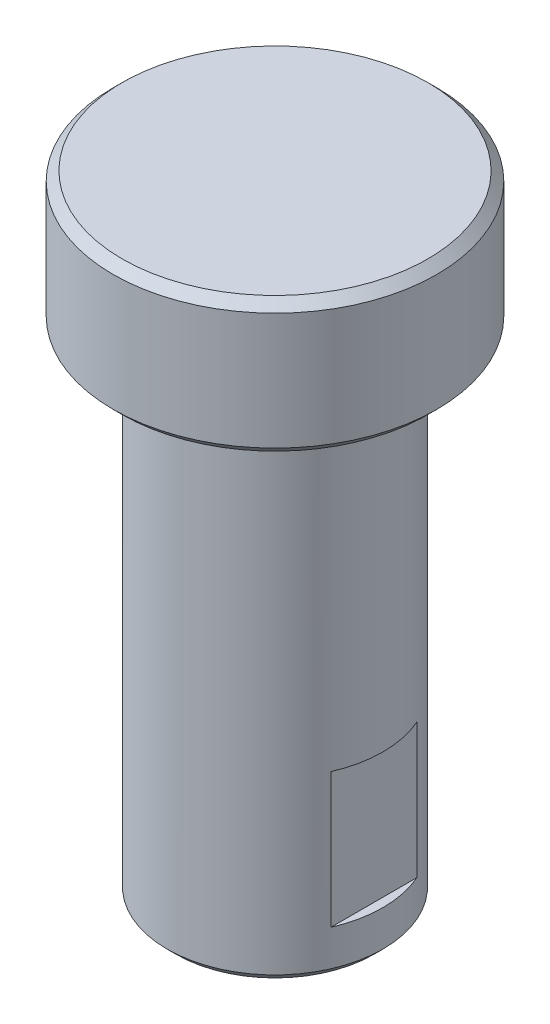
from build123d import *

# Parameters (mm, degrees)
CHAMFER1_SIZE              = 1
CUT_EXTRUDE1_DEPTH         = 55.911039474
CUT_EXTRUDE1_DEPTH_BACK    = 55.911039474
SKETCH3_W                  = 1
SKETCH3_H                  = 15
M14X1_5_TAPPED_HOLE1_D     = 12.5
M14X1_5_TAPPED_HOLE1_DEPTH = 20
M14X1_5_TAPPED_HOLE1_TIP   = 3.755378869


with BuildPart() as part:
    # Sketch2 → Revolve1 (revolve)
    with BuildSketch(Plane.XY, mode=Mode.PRIVATE) as revolve1_sk:
        Polygon((0, 48.654108317), (-18, 48.654108317), (-18, 33.654108317), (-12, 33.654108317), (-12, -21.345891683), (0, -21.345891683), align=None)
    revolve(revolve1_sk.sketch.rotate(Axis((0, 14.106387272, 0), (0, -1, 0)), 270), axis=Axis((0, 14.106387272, 0), (0, -1, 0)))

    # Chamfer1
    chamfer1_edges = [part.edges().sort_by_distance(p)[0] for p in [
        (0, -21.345891683, -12),
        (0, 33.654108317, -18),
        (0, 48.654108317, -18),
    ]]
    chamfer(chamfer1_edges, length=CHAMFER1_SIZE)

    # Sketch3 → Cut-Extrude1 (cut, two sides: drawn at the far end of the back side and taken through both)
    with BuildSketch(Plane.XY.offset(-CUT_EXTRUDE1_DEPTH_BACK)):
        with Locations((-11.5, -8.845891683)):
            Rectangle(SKETCH3_W, SKETCH3_H)
        with Locations((11.5, -8.845891683)):
            Rectangle(SKETCH3_W, SKETCH3_H)
    extrude(amount=CUT_EXTRUDE1_DEPTH + CUT_EXTRUDE1_DEPTH_BACK, mode=Mode.SUBTRACT)

    # M14x1.5 Tapped Hole1
    with Locations(Plane(origin=(0, -21.345891683, 0), x_dir=(-1, 0, 0), z_dir=(0, -1, 0))):
        with Locations((0, 0)):
            Hole(M14X1_5_TAPPED_HOLE1_D / 2, depth=M14X1_5_TAPPED_HOLE1_DEPTH)
            with Locations((0, 0, -(M14X1_5_TAPPED_HOLE1_DEPTH + M14X1_5_TAPPED_HOLE1_TIP / 2))):  # 118° drill point
                Cone(0, M14X1_5_TAPPED_HOLE1_D / 2, M14X1_5_TAPPED_HOLE1_TIP, mode=Mode.SUBTRACT)


solid = part.part
